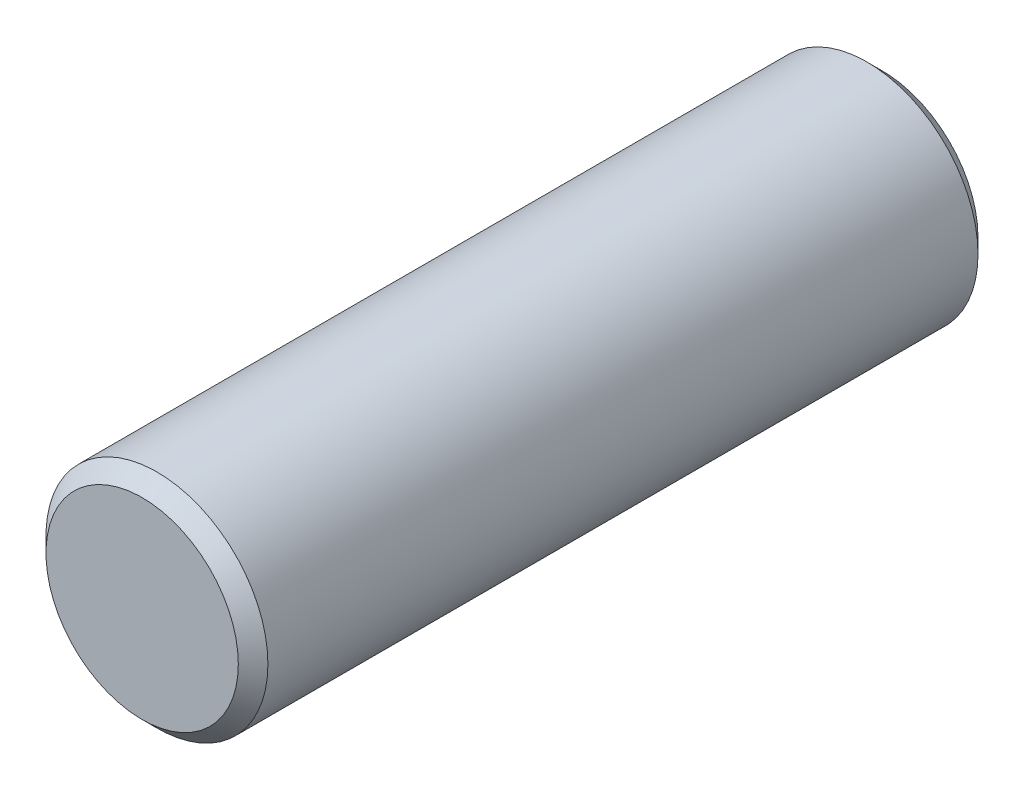
SolidWorks part; units mm, degrees
ref_plane "Front Plane" through (0, 0, 0) normal (0, 0, 1) x (1, 0, 0)
ref_plane "Top Plane" through (0, 0, 0) normal (0, 1, 0) x (1, 0, 0)
ref_plane "Right Plane" through (0, 0, 0) normal (1, 0, 0) x (0, 0, -1)
sketch "Sketch2" plane through (0, 0, 0) normal (0, 0, 1) x (1, 0, 0)
  circle A0 centre (-6.2629, 20.5148) radius 1.5
  dimension "D1" = 3
extrude "Boss-Extrude1" add sketch "Sketch2" against normal blind 10
chamfer "Chamfer1" distance 0.2 angle 45 2 edges at (-4.7629, 20.5148, -10) (-4.7629, 20.5148, 0)
